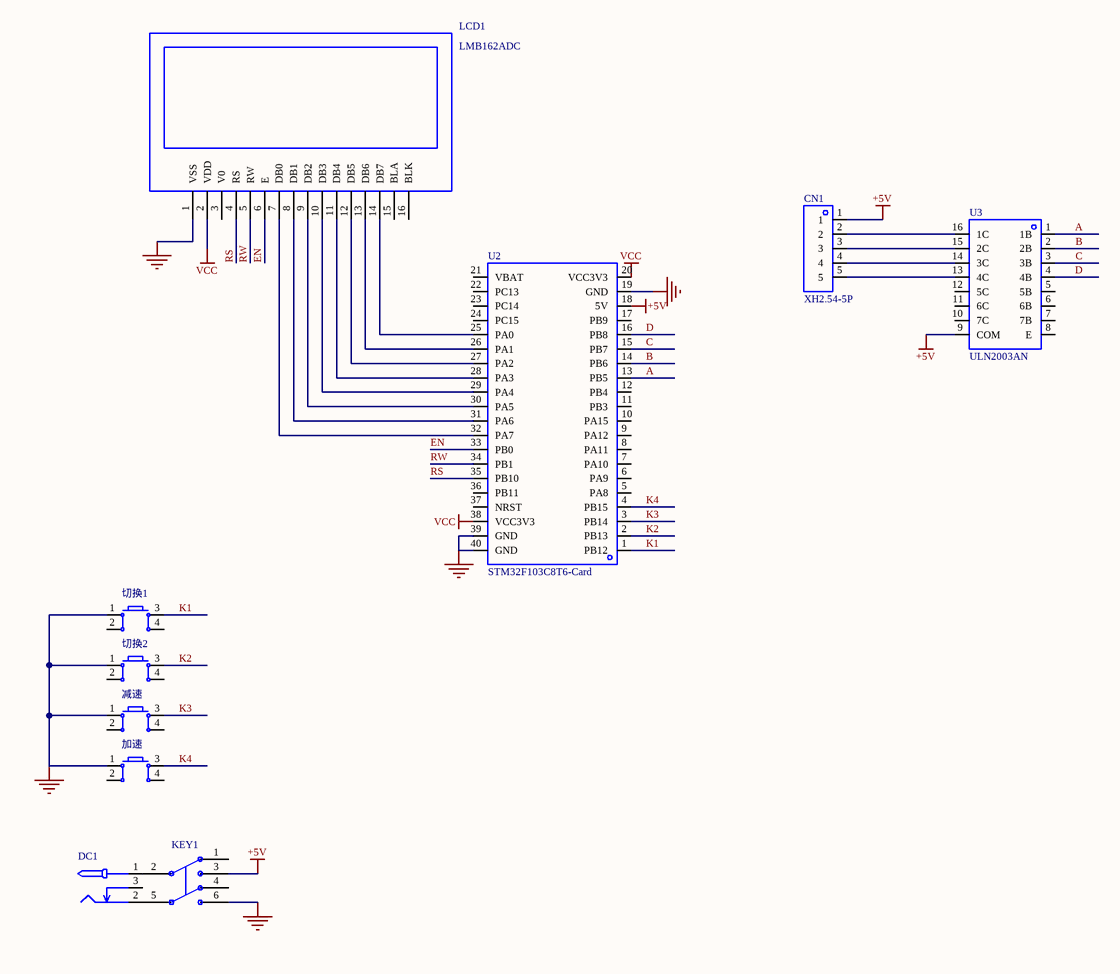
[diagram p0: MISC51167-3.schdoc]
# Altium project MISC51167-2.PrjPcb
1 sheet, 10 parts. Net scope: global (net labels, ports and power ports of the same name join across sheets).
Board file: MISC51167.pcbdoc

## Sheet MISC51167-3.schdoc
size 297 x 209 mm; Version: V1.0; @Project Name: MISC51167; @Page Count: 1; @Update Date: 2025-04-20; @Create Date: 2025-04-20; @Schematic Name: MISC51167; @Page No: 1; @Create Time: 17:38:49; @Update Time: 17:38:49; @Board Name: MISC51167

### Parts
CN1  XH2.54-5P  [CONN-TH_5P-P2.54_C9900008095]
DC1  (no value)  [DC-005_2.5]
KEY1  Non-latching switch 8.5×8.5, silent  [SW-TH_6P-L8.5-W8.5-P2.54]  (value not drawn)
LCD1  LMB162ADC  [LCD1602]
U2  STM32F103C8T6-Card  [CONN-TH_L53.3-W22.9_STM32F103C8T6-CARD]
U3  ULN2003AN  [DIP-16_L19.8-W6.5-P2.54-LS7.6-BL]
减速  (no value)  [SW-TH_4P-L6.0-W6.0-P4.50-LS6.5]
切换1  (no value)  [SW-TH_4P-L6.0-W6.0-P4.50-LS6.5]
切换2  (no value)  [SW-TH_4P-L6.0-W6.0-P4.50-LS6.5]
加速  (no value)  [SW-TH_4P-L6.0-W6.0-P4.50-LS6.5]

### Nets
+5V: CN1.1 KEY1.3 U2.18(5V) U3.9(COM)
GND: KEY1.6 LCD1.1(VSS) U2.19(GND) U2.39(GND) U2.40(GND) 减速.1 切换1.1 切换2.1 加速.1
VCC: LCD1.2(VDD) U2.20(VCC3V3) U2.38(VCC3V3)
A: U2.13(PB5) U3.1(1B)
B: U2.14(PB6) U3.2(2B)
C: U2.15(PB7) U3.3(3B)
D: U2.16(PB8) U3.4(4B)
EN: LCD1.6(E) U2.33(PB0)
K1: U2.1(PB12) 切换1.3
K2: U2.2(PB13) 切换2.3
K3: U2.3(PB14) 减速.3
K4: U2.4(PB15) 加速.3
RS: LCD1.4(RS) U2.35(PB10)
RW: LCD1.5(RW) U2.34(PB1)
NetCN1_2: CN1.2 U3.16(1C)
NetCN1_3: CN1.3 U3.15(2C)
NetCN1_4: CN1.4 U3.14(3C)
NetCN1_5: CN1.5 U3.13(4C)
NetDC1_1: DC1.1 KEY1.2
NetDC1_2: DC1.2 KEY1.5
NetLCD1_7: LCD1.7(DB0) U2.32(PA7)
NetLCD1_8: LCD1.8(DB1) U2.31(PA6)
NetLCD1_9: LCD1.9(DB2) U2.30(PA5)
NetLCD1_10: LCD1.10(DB3) U2.29(PA4)
NetLCD1_11: LCD1.11(DB4) U2.28(PA3)
NetLCD1_12: LCD1.12(DB5) U2.27(PA2)
NetLCD1_13: LCD1.13(DB6) U2.26(PA1)
NetLCD1_14: LCD1.14(DB7) U2.25(PA0)

Not connected (* = marked no-connect by the designer): DC1 3; KEY1 1 4; LCD1 3(V0) 15(BLA) 16(BLK); U2 5(PA8) 6(PA9) 7(PA10) 8(PA11) 9(PA12) 10(PA15) 11(PB3) 12(PB4) 17(PB9) 21(VBAT) 22(PC13) 23(PC14) 24(PC15) 36(PB11) 37(NRST); U3 5(5B) 6(6B) 7(7B) 8(E) 10(7C) 11(6C) 12(5C); 减速 2 4; 切换1 2 4; 切换2 2 4; 加速 2 4

### Notes on the sheet
- 2025-04-20
- Schematic
- Board
- Sheet
- P1
- Drawn
- Reviewed
- Revision
- Size
- A4
- Page 1 of 1

### Library data of the parts
CN1 = XH2.54-5P: Symbol: XH2.54-5P_C9900017328; AddInBom: yes; ModelId: 432b56fff78447668e00d44b84af482c; ModelTransform: 590.55,224.41294,0,0,0,0,0,-21.654,-118.11; Device: XH2.54-5P; LCSC Part Name: XH2.54-5P; SupplierPart: C9900017328; ManufacturerPart: XH2.54-5P; Supplier Footprint: XH2.54-5P; JLCPCB Part Class: Extended library; Supplier: LCSC; ConvertToPcb: yes; FootprintName: CONN-TH_5P-P2.54_C9900008095; ModelName: CONN-TH_5P-P2.54_C9900008095
DC1 = DC-005_2.5: ConvertToPcb: yes; ModelId: f168fe383f964e0ea2af0127ff6ac7b40819f05c4eef4c71ace90d822a990e87; ModelName: DC-IN-TH_DC005; ModelTransform: 366.14,553.15,590.55,90,0,0,137.8,-11.81,-157.48; Device: DC-005_2.5; AddInBom: yes; Supplier Footprint: 插件; SymbolName: DC-005_2.5; FootprintName: DC-005_2.5
KEY1 = 无自锁开关 8.5×8.5 无声: 6 pins, 8.5×8.5; Symbol: No self-locking switch 8.5×8.5 silent; AddInBom: yes; ModelId: 4c72b3966b92446eb355e1bd0fb4f880; ModelTransform: 342.519,334.645,0,180,0,0,0,0,-137.795; Device: Non-latching switch 8.5×8.5, silent; LCSC Part Name: 无自锁开关 8.5×8.5  无声; SupplierPart: C26228; ManufacturerPart: 无自锁开关 8.5×8.5 无声; Supplier Footprint: 插件; JLCPCB Part Class: Extended library; Supplier: LCSC; ConvertToPcb: yes; FootprintName: SW-TH_6P-L8.5-W8.5-P2.54; ModelName: SW-TH_6P-L8.5-W8.5-P2.54
LCD1 = LMB162ADC: 16x2 character LCD module; AddInBom: yes; ModelId: f9d832f46a914cadb50fc4d4cefd2517; ModelTransform: 3149.6,1417.32,0,0,0,0,0,0,-118.11; Symbol: LMB162ADC; Device: LMB162ADC; LCSC Part Name: LMB162ADC; SupplierPart: C9741; ManufacturerPart: LMB162ADC; Supplier Footprint: SIP; JLCPCB Part Class: Extended library; Supplier: LCSC; ConvertToPcb: yes; FootprintName: LCD1602; ModelName: LCD1602
U2 = STM32F103C8T6-Card: AddInBom: yes; Symbol: STM32F103C8T6-CARD; Device: STM32F103C8T6-Card; LCSC Part Name: STM32F103C8T6-Card; SupplierPart: C9900077949; ManufacturerPart: STM32F103C8T6-Card; Supplier Footprint: 插件; Supplier: LCSC; ConvertToPcb: yes; FootprintName: CONN-TH_L53.3-W22.9_STM32F103C8T6-CARD
U3 = ULN2003AN: 通道数:七路;集射击穿电压(Vceo):50V;; Manufacturer: HTC; Symbol: ULN2003AN_C510564; AddInBom: yes; ModelId: 1d8537d07c784a01867ee00a159e9dcc; ModelName: DIP-16_L20.0-W6.4-H3.5-LS7.62-P2.54; ModelTransform: 787.4,311.8104,0,0,0,0,-0.003,0.001,-118.11; number of channels: Seven channels; Collector - Emitter Voltage VCEO: 50V; Voltage - Input(Max): 30V; Device: ULN2003AN; LCSC Part Name: ULN2003AN; SupplierPart: C510564; ManufacturerPart: ULN2003AN; Supplier Footprint: DIP-16; JLCPCB Part Class: Extended library; Datasheet: https://atta.szlcsc.com/upload/public/pdf/source/20200407/C510564_AA23B75C65AE57A24CE05926E39E637A.pdf; Supplier: LCSC; ConvertToPcb: yes; FootprintName: DIP-16_L19.8-W6.5-P2.54-LS7.6-BL; Operating Temperature: -40℃~+85℃
减速 切换1 切换2 加速 = Key_TH_6x6x6: 触点电流:50mA;额定电压(DC):12V;绝缘电阻:100MΩ;电路结构:单刀单掷;安装方式:直插;按钮形状:圆形按钮;按钮/盖帽颜色:黑色;作用力:260gf@±30gf;工作温度:-25℃~+70℃;引脚样式:PC引脚;开关长度:6mm;开关宽度:6mm;开关高度:6mm;带支架:否;; Symbol: Tactile switch; ConvertToPcb: yes; ModelId: 20eee248bc684ccd8cbdbb1d0d91ec6f; ModelName: SW-TH_4P-L6.0-W6.0-H5.0-LS6.5-P4.50; ModelTransform: 236.22,323.03,0,90,0,0,0,0,-137.795; Device: Key_TH_6x6x6; AddInBom: yes; SupplierPart: C2837516; Supplier Footprint: 插件; FootprintName: SW-TH_4P-L6.0-W6.0-P4.50-LS6.5